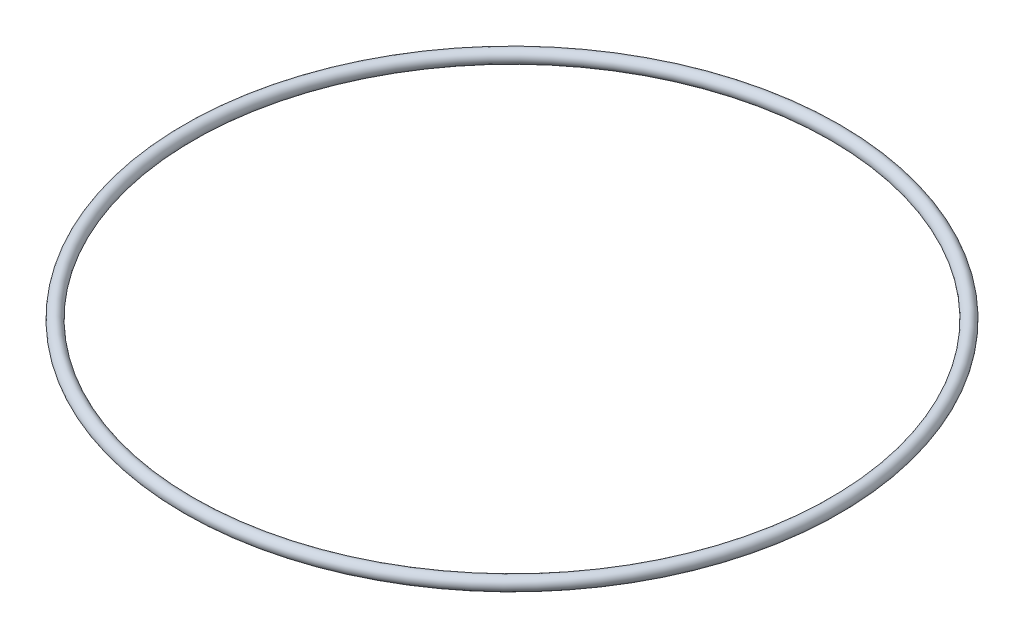
from build123d import *

# Parameters (mm, degrees)
SKETCH1_R = 0.85


with BuildPart() as part:
    # Sketch1 → Revolve1 (revolve)
    with BuildSketch(Plane.XY, mode=Mode.PRIVATE) as revolve1_sk:
        with Locations((-42.85, 0)):
            Circle(SKETCH1_R)
    revolve(revolve1_sk.sketch.rotate(Axis((0, 0, 0), (0, 1, 0)), 270), axis=Axis((0, 0, 0), (0, 1, 0)))


solid = part.part
